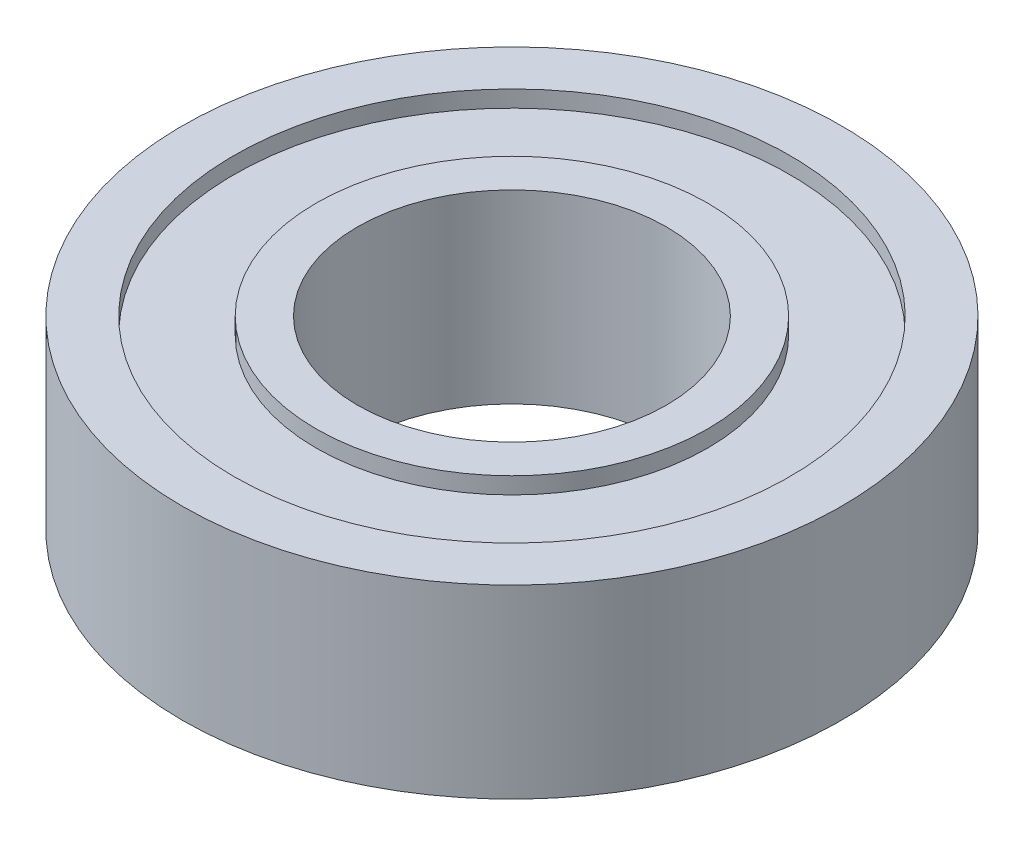
SolidWorks part; units mm, degrees
ref_plane "前视基准面" through (0, 0, 0) normal (0, 0, 1) x (1, 0, 0)
ref_plane "上视基准面" through (0, 0, 0) normal (0, 1, 0) x (1, 0, 0)
ref_plane "右视基准面" through (0, 0, 0) normal (1, 0, 0) x (0, 0, -1)
sketch "草图1" plane through (0, 0, 0) normal (0, 0, 1) x (1, 0, 0)
  line L0 (7.5, 0) -> (7.5, -9)
  line L1 (7.5, 0) -> (9.5, 0)
  line L2 (9.5, 0) -> (9.5, -0.8072)
  line L3 (9.5, -0.8072) -> (13.5, -0.8072)
  line L4 (13.5, 0) -> (16, 0)
  line L5 (13.5, -0.8072) -> (13.5, 0)
  line L6 (16, 0) -> (16, -9)
  line L7 (7.5, -9) -> (9.5, -9)
  line L8 (9.5, -9) -> (9.5, -8)
  line L9 (9.5, -8) -> (13.5, -8)
  line L10 (13.5, -8) -> (13.5, -9)
  line L11 (13.5, -9) -> (16, -9)
  line L12 (0, 13.4383) -> (0, -11.1054) construction
  dimension "D1" = 7.5
  dimension "D2" = 2
  dimension "D3" = 16
  dimension "D4" = 9
  dimension "D5" = 9
  dimension "D6" = 4
  dimension "D7" = 4
  dimension "D8" = 1
revolve "旋转1" add sketch "草图1" angle 360 about L12
